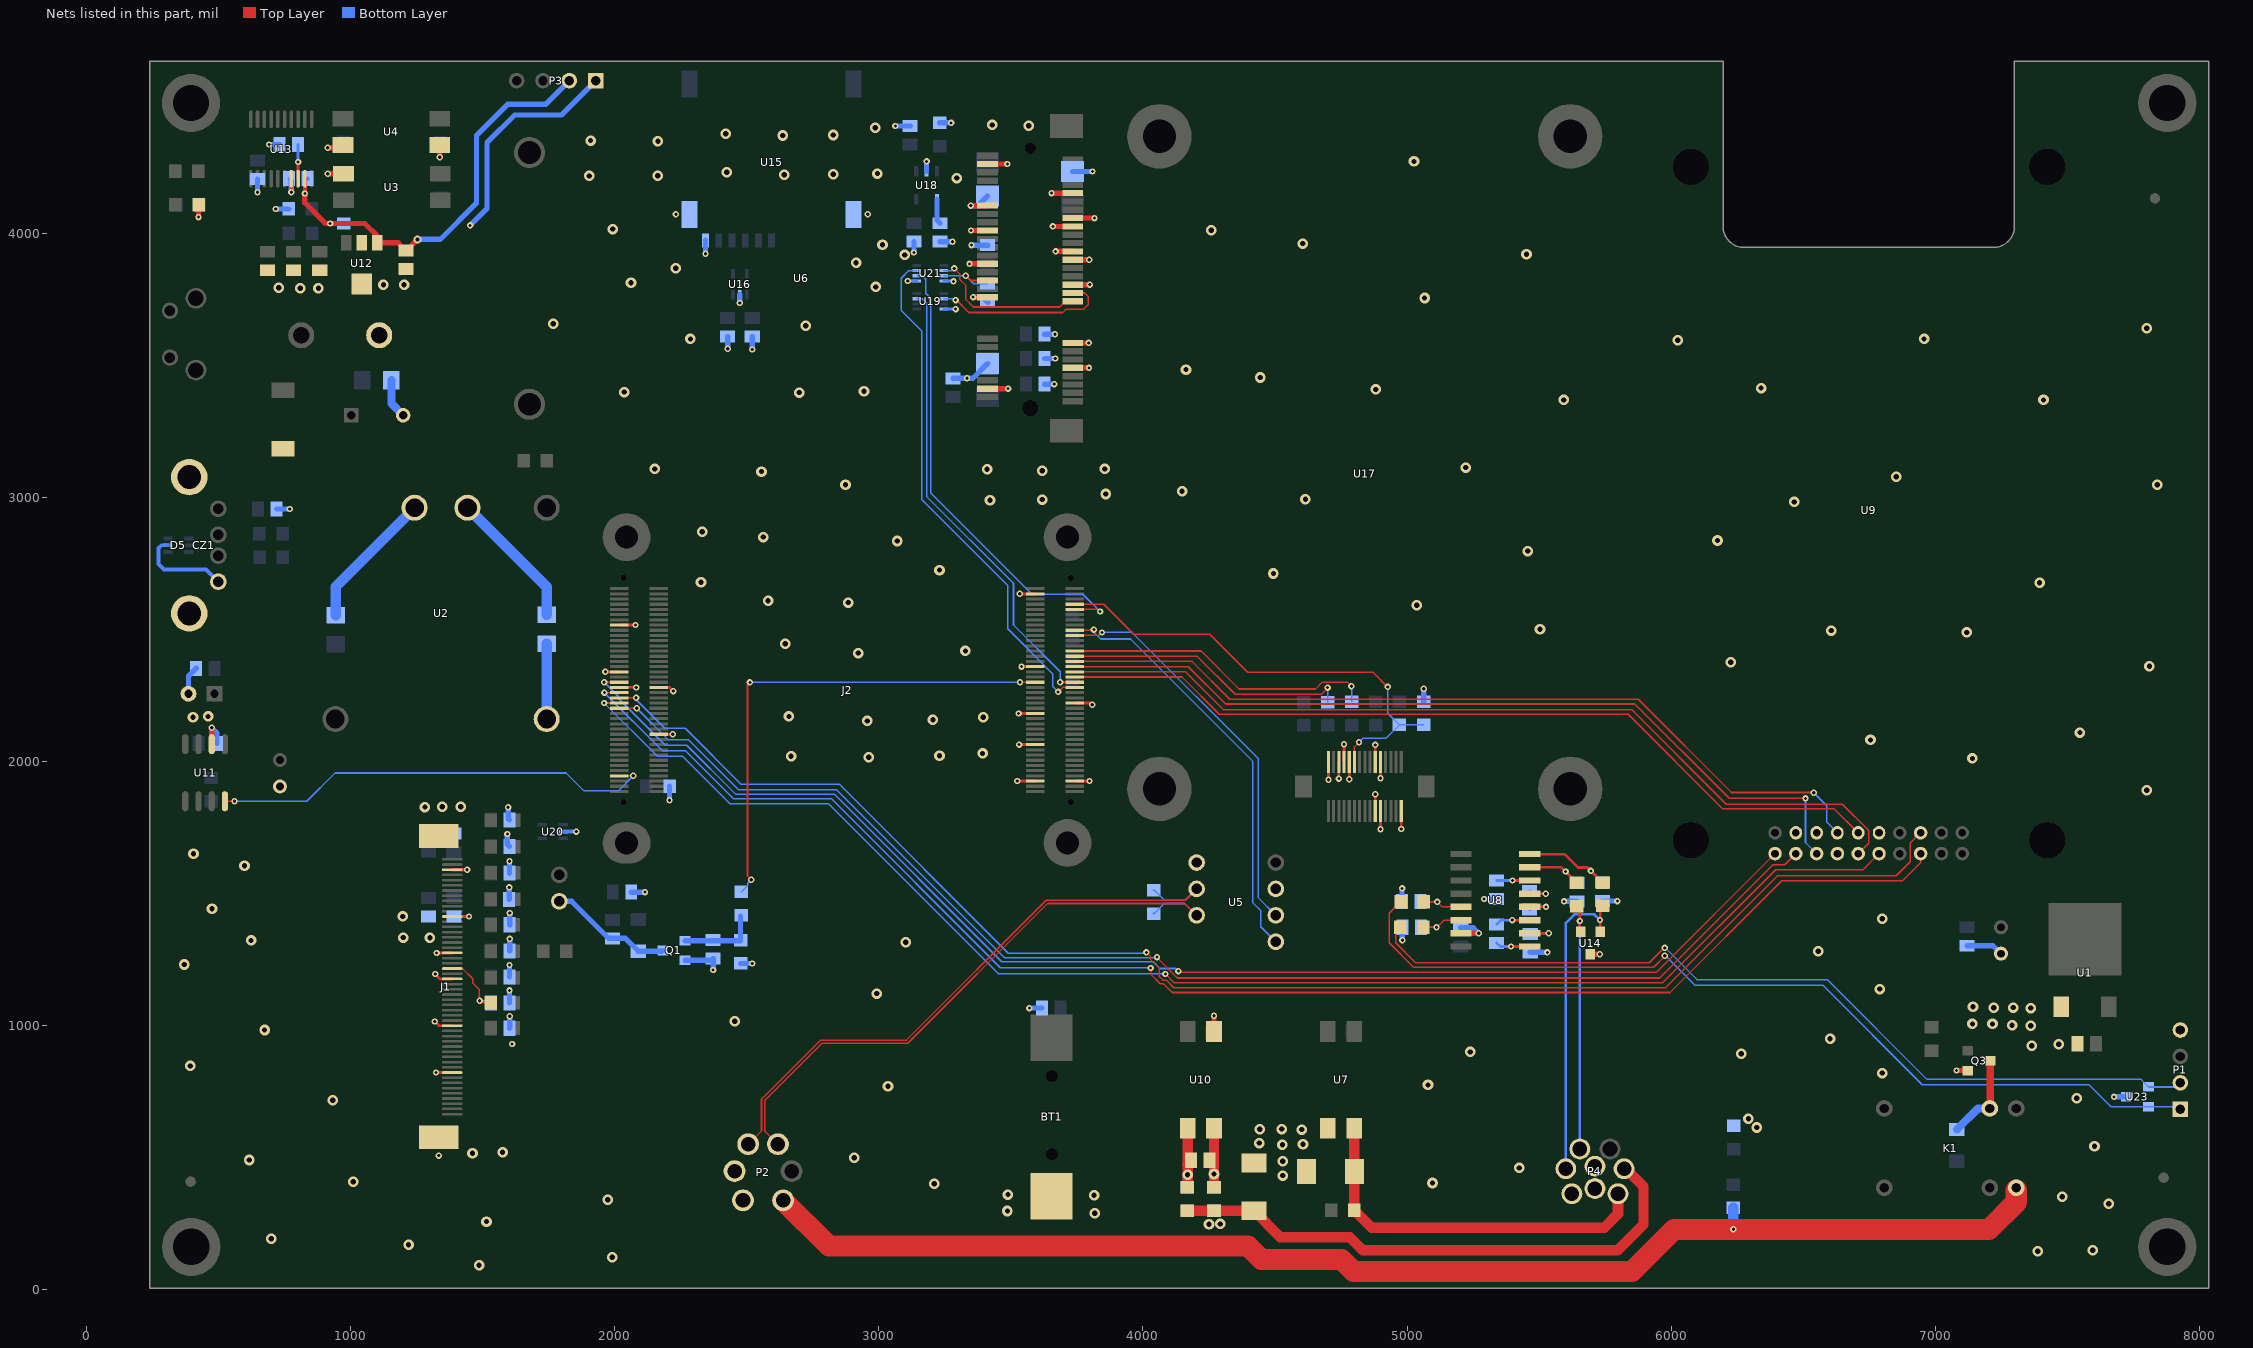
[diagram p0: the nets of this part, all layers, seen from the top]
# Altium PCB MISC82794.PcbDoc (part 3 of 5)
Units mil, origin at the board's own origin, x right, y up, seen from the top; angles counter-clockwise.
Board outline 7795.28 x 4645.67 mil, 4 copper layers (Top Layer, GND, POWER, Bottom Layer); 157 components, 133 nets, 768 pads, 456 vias.

## Part data
BT1: library part 1.10.05.0096, "2P,pitch 1.25mm,wafer with slotted frame,90°,FPC2-49T"
BZ1: library part 1.06.09.0016, "AS-905I-LF,passive,Ф9×4.8mm,Changzhou Lixiang,RoHS"
C1 C6 C27 C36 C47 C48 C49: library part 1.02.11.0018, "220μF,16V,Ф6.3×7mm,,Zhuhai Huaguan,RoHS"
C2 C4 C5 C18 C23 C30 C31 C32 C33 C34 C35 C37: library part "Cap Semi", "Capacitor (Semiconductor SIM Model)"
C3 C7 C13 C19 C22 C24 C26 C29 C50 C51 C52 C53 C54 C55 C56 C57: library part 1.02.17.0020, "0.1μF,±10%,X5R,25V,0402,RoHS"
C8 C9 C10 C11 C12: library part 1.02.17.0005, "15PF,±5%,50V,COG,0402,RoHS"
C14 C15 C16 C17: library part 1.02.17.0021, "1nF,CAP,CER,1000PF,50V,CDG,GRM1555C1H102JA01D,0402,MURATA,RoHS"
C20: library part 1.02.01.0065, "10uF,6.3V,X5R,GRM188R60J106ME47D,0603,Murata,RoHS"
C21 C28: library part 1.02.02.0055, "106,10μF,±10%,10V,X5R,0805,RoHS"
C25 C38 C39 C40 C41 C42 C43 C44 C61 C62: library part Cap, "Capacitor"
C58 C59: library part 1.02.17.0020, "1uF,±10%,X7R,25V"
C60: library part 1.02.17.0020, "22nF,±10%,X5R,50V"
CZ1: library part 1.10.12.0012, "3190004-H73-R,USB-A receptacle,vertical,90°,THT,WCON,RoHS"
D1: library part 1.04.07.0027, "1N4148,SOD-323,RoHS"
D3 D4: library part "D Zener", "Zener Diode"
D5: library part 1.05.10.0376, "NUP4202W1T2G,SC-88,ON,RoHS"
D10: library part Diode, "Default Diode"
DD1 DD2: library part LED_0
J1: library part 1.10.01.0028, "Data connector,0.5FFC-50,SMD,bottom contact,RoHS"
J2: "DF12D(3.0)-80DP-0.5V(81),Fmale,SMT,HRS,RoHS"
K1: library part Relay-SPDT, "Single-Pole Dual-Throw Relay"
L1: library part 1.03.03.0022, "BM02Y190S40R,0402,Fengjing,RoHS"
L2: library part Inductor, "Inductor"
P1 P3: library part "Header 4", "Header, 4-Pin"
P2: library part "Header 6", "Header, 6-Pin"
P4: library part "Header 8", "Header, 8-Pin"
Q1 Q3: library part 1.04.09.0001, "SS8050LT(1.5A),SOT-23,JCET,RoHS"
R1 R8 R11 R29 R30 R31 R32 R33 R34 R35 R36 R37 R38 R41 R42 R43 R44 R46 R47 R48: library part RES
R2 R3 R4 R5 R6 R25 R26: library part 1.01.17.0023, "22Ω,±5%,0402,RALEC,RoHS"
R9 R10: library part 1.01.17.0019
R12 R13 R14 R15: library part 1.01.17.0004, "0Ω,±5%,0402,RALEC,RoHS"
R16: library part "Res Varistor", "Varistor (Voltage-Sensitive Resistor)"
R17 R18 R19 R20 R21 R22 R23 R28 R49 R50: library part 1.01.17.0004
R24 R27 R39 R40 R45: library part 1.01.17.0006, "10K,±5%,0402,RALEC,RoHS"
S1: "6×6×5.0mm,black,SMD,,*"
U1 U12: library part VOLTREG1
U2: library part E2403UHBDD-10W
U3 U4 U7 U10: library part TLP281-1, "Optoisolator"
U8: library part SP202ECT
U9: library part OEMStar, "OEMStar"
U11: library part 1.05.09.0064
U14 U23: library part PESD12VL2BT
U16 U20: library part 1.05.10.0265, "PESD3V3L4UG,SOT-353,NXP,RoHS"
U18: library part RT9193, "RT9193"

## Free pads (board coordinates)
  round 39.37 smd mask+39.37: 0(395,410) 0(7831,4132) 0(7864,425)
  round 39.37 smd far side mask+39.37: 0(395,410) 0(7831,4132) 0(7864,425)

## Via types
v1: diameter 24, hole 12, Top Layer to Bottom Layer, 258 vias
v2: diameter 40, hole 20, Top Layer to Bottom Layer, 197 vias
v3: diameter 30, hole 15, Top Layer to Bottom Layer, 1 vias

## Nets (pads, with @x,y where several pads share a name; then routed paths per layer and width w, separated by ;. In a path a pad name is that pad's centre, name@x,y a point inside that pad or via, vN(x,y) a via of type N, cw(c..) or ccw(c..) an arc to the next point about the centre after c; other vN are vias at no path point)
5V: C32.1 C35.1 P3.2 R33.1 U12.1 U13.9 | length 1711.3
  Top Layer w15: v1(827.57,4150.57) U13.9@827.57,4206.79
  Top Layer w20: v1(827.57,4150.57) 827.57,4115.43 906,4037 1054,4037 1102,3989 U12.1@1102,3964.3 1180.7,3964.3 C32.1@1211,3934 v3(1254,3977)
  Bottom Layer w15: v1(827.57,4150.57) 827.57,4197.39 C35.1@836.98,4206.79
  Bottom Layer w20: v1(923,4037) R33.1@975,4037 ; v3(1254,3977) 1340,3977 1477,4114 1477,4370 1595,4488 1739,4488 P3.2@1829,4578
232RX0: P4.5 R38.1 U14.1 | length 1184.7
  Top Layer w10: U14.1@5731.4,1355.5 5731.4,1445.4 R38.1@5740,1454
  Bottom Layer w10: P4.5@5600.76,458.69 5600.76,1389.76 5633,1422 5708.4,1422 v1(5730,1400.4)
232RX1: P1.1 R48.1 U23.2 | length 3491.8
  Top Layer w6: R48.1@4954,1469 R48.1@4975,1469 4932,1426 4932,1314 5024,1222 5934,1222 5976,1264 5976,1270 5973,1267 v1(5975,1265)
  Bottom Layer w6: v1@5981,1262 6089,1154 6573,1154 6950,777 7581,777 7664.4,693.6 U23.2@7806.5,693.6 7917.4,693.6 P1.1@7927,684
232TX0: P4.4 R35.1 U14.2 | length 966.6
  Top Layer w10: R35.1@5643,1453 5654,1442 5654,1358.1 U14.2@5656.6,1355.5
  Bottom Layer w10: P4.4@5653.91,533.49 5653.91,629 v1(5653.91,1396.91)
232TX1: P1.2 R47.1 U23.1 | length 3329.1
  Top Layer w6: R47.1@4974,1373 4957,1356 4957,1314 5032,1239 5917,1239 5973.8,1295.8 v1@5973.8,1297.5 ; v1@5974.5,1297.5 v1@5973.8,1297.5 ; v1(5975,1295) 5975,1298.6 5973.8,1299.8 v1@5973.8,1297.5
  Bottom Layer w6: v1@5972,1300 6097,1175 6590,1175 6968,797 7777.9,797 U23.1@7806.5,768.4 7911.4,768.4 P1.2@7927,784
433_M0: J2.B73 R49.1 R50.1 U17.11 | length 1831
  Top Layer w6: J2.B73@3742.2,2595.8 3851.2,2595.8 3965,2482 4253,2482 4397,2338 4871,2338 v1@4927,2282 ; U17.11@4800.63,1998.52 4800.63,2055.63 v1(4818,2073)
  Bottom Layer w6: v1(4818,2073) 4833,2088 4920,2088 R49.1@4971,2139 ; v1(4927,2283) 4927,2183 R49.1@4971,2139 ; R50.1@5063,2139 R49.1@4971,2139
433_RX: J2.B53 R42.1 | length 1100.4
  Top Layer w6: J2.B53@3742.2,2398.95 4205.05,2398.95 4349,2255 4676,2255 4699,2278 v1@4699,2285
  Bottom Layer w6: v1(4699,2280) 4699,2285 4700,2286 R42.1@4700,2225
433_TX: J2.B55 R43.1 | length 1202
  Top Layer w6: J2.B55@3742.2,2418.64 4220.36,2418.64 4364,2275 4653,2275 4679,2301 4774,2301 4784,2291 4784,2285 4790,2285 v1@4789,2284 ; v1@4789,2279 v1(4789,2285)
  Bottom Layer w6: v1@4789,2279 v1(4789,2285) ; v1@4789,2284 4790,2285 R43.1@4790,2226
BOOM_SEN: D4.2 P4.2 R19.1 R20.1 | length 2074.7
  Top Layer w39.37: R20.1@4167,300 4167.55,299.45 D4.2@4421,299.45 4520.45,200 4783,200 4832,151 5798,151 5895,248 5895,391 5827.31,458.69 P4.2@5821.24,458.69
BUZZER: J2.B44 R9.1 | length 1898.7
  Top Layer w6: v1(2512,2300.06) 2503,2291.06 2503,1567 v1(2517,1553) ; v1(3534.47,2300.53) J2.B44@3592.6,2300.53
  Bottom Layer w6: R9.1@2480,1507 2504,1531 2504,1540 v1(2517,1553) ; v1(2512,2300.06) 2512.47,2300.53 v1(3534.47,2300.53)
CAN0_RXD: J2.B63 U5.1 | length 1605
  Top Layer w6: J2.B63@3742.2,2497.38 v1@3814.38,2497.38
  Bottom Layer w6: v1(3814.38,2499.62) 3814.38,2489.92 3840.3,2464 3953,2464 4415,2002 4415,1467 4446,1436 4446,1375 U5.1@4503,1318
CAN0_TXD: J2.B61 U5.2 | length 1517.8
  Top Layer w6: J2.B61@3742.2,2477.69 3833.69,2477.69 v1(3845,2489)
  Bottom Layer w6: v1(3845,2489) 3959,2489 4437,2011 4437,1484 U5.2@4503,1418
CANH0: P2.3 R32.1 U5.7 | length 2346
  Top Layer w6: P2.3@2618.3,551.81 2568,602.11 2568,717 2785,934 3110,934 3639,1463 4158,1463 U5.7@4203,1418
  Bottom Layer w6: R32.1@4040,1425 4042.4,1425 4080.4,1463 4158,1463 U5.7@4203,1418
CANL0: P2.4 R32.2 U5.6 | length 2364.3
  Top Layer w6: P2.4@2505.7,551.81 2556,602.11 2556,721.97 2780.03,946 3105.03,946 3634.03,1475 4160,1475 U5.6@4203,1518
  Bottom Layer w6: R32.2@4040,1513 4044,1513 4082,1475 4160,1475 U5.6@4203,1518
CTRL_12V: K1.2 P2.1 R39.2 | length 5014.5
  Top Layer w80: P2.1@2637.98,339.21 2811.2,166 4398,166 4449,115 4752,115 4797,70 5851,70 6010,229 7203,229 7306,332 K1.2@7306,377.4
  Bottom Layer w40: v1(6235,230) R39.2@6235,311
EN_USB0: J2.A73 U11.4 | length 1695
  Top Layer w6: U11.4@525,1849.97 v1@560.97,1849.97 ; J2.A73@2017.8,1946.2 v1(2070.8,1946.2)
  Bottom Layer w6: v1(561,1850) 835,1850 942,1957 1816,1957 1884,1889 2013.61,1889 v1(2070.8,1946.2)
GND: BT1.2 C1.2 C2.2 C3.2 C5.2 C6.2 C8.2 C9.2 C10.2 C11.2 C12.2 C13.1 C14.2 C15.2 C16.2 C17.2 C19.1 C20.1 C21.2 C22.1 C24.2 C26.1 C27.2 C28.2 C29.2 C37.2 C39.2 C40.2 C42.2 C43.2 C44.2 C47.2 C48.2 C49.2 C50.2 C51.2 C52.2 C53.2 C54.1 C55.1 C56.2 C57.2 C58.1 C59.1 C60.1 C61.1 C62.1 CZ1.4 D5.2 DD1.2 J1.3 J1.12 J1.19 J1.24 J1.33 J1.42 J1.51 J1.52 J2.A15 J2.A33 J2.A39 J2.A40 J2.A58 J2.B5 J2.B6 J2.B20 J2.B32 J2.B35 J2.B50 J2.B78 P1.4 P4.6 Q1.2 Q3.2 R10.1 R27.1 R46.2 R50.2 U1.1 U2.5 U4.3 U5.3 U6.4 U6.9 U6.15 U6.18 U6.21 U6.26 U6.27 U6.29 U6.34 U6.35 U6.37 U6.40 U6.43 U6.50 U8.15 U9.10 U9.13 U9.16 U9.18 U10.3 U11.6 U14.3 U15.5 U15.8 U15.9 U16.2 U17.1 U17.5 U17.7 U17.9 U17.19 U17.20 U17.21 U17.22 U17.30 U18.2 U19.4 U20.2 U21.4 U21.5 U23.3 | length 6377.2
  Top Layer w10: v1(1319,1016) 1334.8,1000.2 J1.33@1385.39,1000.2 ; v1(1321,1196) 1339.63,1177.37 J1.24@1385.39,1177.37 ; v1(1324.04,823.04) J1.42@1385.39,823.04 ; v1(1326.2,1275.8) J1.19@1385.39,1275.8 ; J1.12@1385.39,1413.59 v1(1448.59,1413.59) ; J2.A39@2017.8,2280.84 v1(2081.84,2280.84) ; J2.A58@2167.4,2103.68 v1(2220.32,2103.68) ; J2.A40@2167.4,2280.84 2208.16,2280.84 v1(2222,2267) ; v1(4702.2,1931.2) U17.1@4702.2,1998.52 ; v1(4741.57,1935.57) U17.5@4741.57,1998.52 ; U17.7@4761.26,1998.52 v1(4761.26,2065.74) ; v1(4780.94,1933.06) U17.9@4780.94,1998.52
  Top Layer w11: v1(1965.1,2339.9) J2.A33@2017.8,2339.9 ; J2.A15@2017.8,2517.06 v1(2079.06,2517.06) ; v1(3524.51,1926.51) J2.B6@3592.6,1926.51 ; v1(3529.42,2182.42) J2.B32@3592.6,2182.42 ; v1(3531.31,2064.31) J2.B20@3592.6,2064.31 ; v1(3533.83,2635.17) J2.B78@3592.6,2635.17 ; v1(3540.58,2359.58) J2.B50@3592.6,2359.58 ; J2.B5@3742.2,1926.51 v1(3797.49,1926.51) ; J2.B35@3742.2,2221.79 3801.21,2221.79 v1(3808,2215) ; U17.20@4879.37,1813.48 v1(4879.37,1876.37) ; U17.19@4879.37,1998.52 v1(4879.37,2063.37) ; v1(4899.06,1744.06) U17.22@4899.06,1813.48 ; v1(4899.06,1936.94) U17.21@4899.06,1998.52 ; v1(4977.8,1745.2) U17.30@4977.8,1813.48
  Top Layer w12: J1.3@1385.39,1590.76 v1(1441.76,1590.76)
  Top Layer w20: v1(425.14,4061.14) DD1.2@425.14,4108.86 ; U11.6@475,2066.03 v1(475,2128) ; v1(1338.07,4288.07) U4.3@1338.07,4334 ; v1(3343.24,3884.24) U6.26@3411.58,3884.24 ; v1(3348.28,4104.72) U6.40@3411.58,4104.72 ; v1(3349.23,4010.23) U6.34@3411.58,4010.23 ; v1(3357.26,3758.26) U6.18@3411.58,3758.26 ; U6.4@3411.58,3411.8 v1(3489.8,3411.8) ; U6.50@3411.58,4262.2 v1(3486.8,4262.2) ; v1(3654.04,4151.96) U6.43@3734.42,4151.96 ; v1(3659.02,4025.98) U6.35@3734.42,4025.98 ; v1(3669.51,3931.49) U6.29@3734.42,3931.49 ; U6.9@3734.42,3490.54 v1(3795.54,3490.54) ; U6.15@3734.42,3585.03 v1(3794.97,3585.03) ; U6.21@3734.42,3805.5 v1(3798.5,3805.5) ; U6.27@3734.42,3899.99 v1(3796.99,3899.99) ; U6.37@3734.42,4057.47 v1(3816.47,4057.47) ; U10.3@4269,978.07 v1(4269,1038) ; U8.15@5204,1350 v1(5271,1350) ; U14.3@5694,1270.5 v1(5729.5,1270.5) ; v1(7079.4,830.6) Q3.2@7122.5,830.6
  Bottom Layer w10: U21.4@3246.18,3819.47 3281.53,3819.47 v1(3283,3818)
  Bottom Layer w11: v1(3109.47,3819.47) U21.5@3143.82,3819.47 ; U19.4@3246.45,3712.94 v1(3290.94,3712.94)
  Bottom Layer w15: D5.2@309.55,2819 285,2819 274,2808 274,2748 294,2728 453.32,2728 CZ1.4@500.12,2681.2 ; U20.2@1805.45,1735 v1(1855,1735)
  Bottom Layer w20: C27.2@386.79,2257 386.79,2323.79 C28.2@416,2353 ; v1(475,2128) 495,2108 C26.1@495,2069 ; C29.2@720,2956 v1(770,2956) ; v1(1594,1726) 1594,1686.6 C15.2@1602,1678.6 ; v1(1597,1827) 1597,1783.6 C17.2@1602,1778.6 ; C14.2@1601,1478.6 v1(1601,1524) ; C11.2@1602,990.6 1603,991.6 v1(1603,1036) ; C10.2@1602,1086.6 v1(1602,1134) ; C12.2@1602,1184.6 v1(1602,1230) ; C16.2@1602,1577.6 v1(1602,1623) ; C9.2@1603,1283 v1(1603,1329) ; C8.2@1603,1382.6 v1(1603,1427) ; C3.2@2063,1506 v1(2115,1506) ; v1(2208,1854) R27.1@2208,1907 ; Q1.2@2266.5,1247.6 C13.1@2366.6,1247.6 ; v1(2344.39,3922.39) U15.5@2344.39,3973.23 ; v1(2373,1211) C13.1@2373,1254 ; v1(2428,3563) C55.1@2428,3609 ; v1(2474,3736) U16.2@2474,3767.55 ; R10.1@2478,1236 v1(2521,1236) ; v1(2521,3560) C54.1@2521,3609 ; v1(3063,4406) C59.1@3119,4406 ; v1(3133,3927) C58.1@3133,3968 ; U18.2@3181,4235.15 v1(3181,4272) ; R46.2@3230,4418 v1(3274,4418) ; C60.1@3232,3968 v1(3279,3968) ; C57.2@3281,3451 v1(3334,3451) 3356.01,3451 C48.2@3412,3506.99 ; v1(3348.28,4104.72) 3374.71,4104.72 C47.2@3411,4141.01 ; v1(3351,3955) C56.2@3412,3955 ; v1(3357.26,3758.26) 3392.74,3758.26 C53.2@3412,3739 ; v1(3570,1067) C24.2@3618,1067 ; C50.2@3627,3429 v1(3664,3429) ; C51.2@3627,3526 v1(3668,3526) ; C52.2@3627,3618 v1(3667,3618) ; C49.2@3734,4233.99 v1(3808.99,4233.99) ; C62.1@4981,1470 v1(4981,1520) ; v1(4982,1324) C61.1@4982,1373 ; R50.2@5063,2227 v1(5063,2276) ; C39.2@5203,1371 5250,1371 v1(5271,1350) ; v1(5291,1480) C42.2@5339,1480 ; C40.2@5466,1278 v1(5531,1278) ; v1(5594,1471) C44.2@5643,1471 ; C43.2@5740,1472 v1(5796,1472) ; C5.2@7120,1303 7218,1303 C1.2@7248,1273 ; v1(7676,731) U23.3@7721.5,731
  Bottom Layer w40: U2.5@1743,2161 C37.2@1743,2445.88
  other v1: 1334.61,508.39 1612,931 2231.85,4071.85 2958.15,4071.85
  other v2: 1487,94 1991,124 7387,147 7595,150 1220,171 700,194 1515,259 3818,290 3487,299 7656,326 1974,342 7480,353 3815,359 3489,361 3210,402 5096,405 1011,410 5425,462 617,492 2907,500 1462,518 1576,521 7602,544 933,718 7535,726 3035,771 5079,776 6799,821 394,848 6265,894 5239,901 7364,924 7467,930 6601,951 675,984 7361,1000 7290,1002 7140,1007 7216,1007 2455,1017 7361,1067 7221,1068 7295,1069 7142,1072 2992,1122 6789,1139 371,1232 6556,1282 3102,1316 624,1323 1301,1333 1200,1334 6799,1405 1198,1414 476,1443 599,1606 406,1651 1282,1828 1348,1829 1418,1829 7800,1892 7140,2012 2962,2017 2668,2020 3230,2022 3393,2031 6754,2082 7547,2110 2956,2154 3205,2159 404,2168 3396,2168 461,2171 2660,2171 7810,2361 6225,2376 2922,2411 3328,2419 2646,2446 7118,2489 6606,2496 5503,2501 5036,2592 2884,2602 2581,2609 7394,2677 2327,2679 4494,2712 3230,2725 5457,2797 3070,2835 6175,2837 2563,2850 2332,2870 6466,2983 3421,2989 3619,2992 4615,2993 3859,3013 4148,3023 2874,3048 7840,3048 6852,3078 2556,3098 3619,3101 3410,3107 2152,3108 3855,3108 5222,3113 5593,3369 7409,3369 2699,3397 2036,3399 2944,3402 4881,3409 6340,3414 4444,3454 4163,3484 6024,3595 2287,3600 6957,3600 7800,3640 2724,3650 1768,3658 5066,3755 2989,3797 2062,3813 2231,3868 2914,3888 3098,3918 5452,3921 3014,3957 4605,3961 4259,4011 1993,4016 3295,4209 1904,4217 2163,4218 2642,4221 2828,4223 2995,4226 2425,4231 5026,4272 2164,4348 1909,4351 2637,4370 2828,4372 2421,4377 2987,4399 3568,4407 3430,4410
GND1: C18.2 C23.1 C30.2 C31.2 C32.2 C33.1 C34.1 C35.2 C36.2 C37.1 CZ1.5 CZ1.6 D3.1 D4.1 P2.5 P2.6 P3.1 P4.7 P4.8 R16.1 R23.2 R34.1 R40.2 U2.2 U3.3 U4.2 U5.5 U7.3 U12.2 U13.7 | length 1898.1
  Top Layer w12: v1(776.39,4155.39) U13.7@776.39,4206.79
  Top Layer w20: v1(914,4225) U3.3@973.93,4225 ; v1(914,4324) 961.93,4324 U4.2@971.93,4334
  Bottom Layer w12: C35.2@766.98,4206.79 C35.2@776.39,4197.38
  Bottom Layer w20: v1(648,4155) C34.1@648,4205 ; v1(692,4336) C33.1@732,4336 ; v1(717,4092) R34.1@766,4092 ; v1(776.39,4155.39) C35.2@776.39,4197.38 ; v1@1453,4029 v1(1453,4030) 1517,4094 1517,4343 1622,4448 1799,4448 P3.1@1929,4578
  Bottom Layer w30: C23.1@1155.12,3444 1155.12,3355.31 C36.2@1199.43,3311
  Bottom Layer w40: U2.2@1443,2961 1743,2661 C37.1@1743,2556.12
  other v2: 4250,249 4293,250 4529,433 4529,487 4528,550 4606,552 4440,556 4601,607 4442,608 4525,609 6324,615 6292,648 810,3792 879,3792 729,3794 1125,3805 1203,3805
GND_SPD: D3.2 P4.1 R17.1 U7.4 | length 1433.2
  Top Layer w40: U7.4@4800,611.93 R17.1@4800,302 4866,236 5746,236 5798.4,288.4 P4.1@5798.4,364.2
GPS_EVT1: J2.A45 U9.9 | length 5525.6
  Top Layer w6: v1(1960.21,2221.79) J2.A45@2017.8,2221.79 ; v1(4085,1196) 4118,1163 5967,1163 6395,1591 6725.58,1591 U9.9@6786.39,1651.8
  Bottom Layer w6: v1(1960.21,2221.79) 2161,2021 2256,2021 2437,1840 2810,1840 3453,1197 4082,1197 4084,1195 v1(4085,1196)
GPS_PPS: J2.A37 U9.19 | length 5129.9
  Top Layer w6: v1(1960.47,2300.53) J2.A37@2017.8,2300.53 ; v1@4138,1202 5942.88,1202 U9.19@6392.69,1651.8
  Bottom Layer w6: v1(1960.47,2300.53) 2014,2247 2014,2240 2192,2062 2273,2062 2458,1877 2831,1877 3466,1242 4040,1242 4065,1217 4124,1217 v1(4134,1207) v1@4134,1206
GPS_PV: J2.A47 U9.17 | length 5070.8
  Top Layer w6: J2.A47@2017.8,2202.1 v1(2083.9,2202.1) ; v1(4053,1260) 4053,1258.3 4130.3,1181 5956,1181 6385,1610 6429.62,1610 U9.17@6471.43,1651.8
  Bottom Layer w6: v1(2083.9,2202.1) 2204,2082 2281,2082 2469,1894 2840,1894 3477,1257 v1@4050,1257
GPS_RST: J2.A41 U9.5 | length 5760.7
  Top Layer w6: v1(1961.16,2261.16) J2.A41@2017.8,2261.16 ; v1(4029,1219) 4029,1196 4066,1159 4078,1159 4111,1126 5995,1126 6418,1549 6875,1549 6943.87,1617.87 U9.5@6943.87,1651.8
  Bottom Layer w6: v1(1961.16,2261.16) 2181.32,2041 2268,2041 2449,1860 2820,1860 3460,1220 4028,1220 v1(4029,1219)
GPS_RX1: J2.B45 U9.12 | length 3209.7
  Top Layer w6: J2.B45@3742.2,2320.21 4147.79,2320.21 4289,2179 5837,2179 6195,1821 6617.19,1821 U9.12@6707.65,1730.54
GPS_RX2: J2.B49 U9.15 | length 3199
  Top Layer w6: J2.B49@3742.2,2359.58 4171.42,2359.58 4313,2218 5862,2218 6219,1861 v1(6508,1861)
  Bottom Layer w6: v1(6508,1861) 6508,1693.97 U9.15@6550.17,1651.8
GPS_TX1: J2.B47 U9.11 | length 3357.4
  Top Layer w6: J2.B47@3742.2,2339.9 4161.1,2339.9 4304,2197 5850,2197 6208,1839 6647.29,1839 6747,1739.29 6747,1691.16 U9.11@6707.65,1651.8
GPS_TX2: J2.B51 U9.14 | length 3192.1
  Top Layer w6: J2.B51@3742.2,2379.27 4185.73,2379.27 4329,2236 5875,2236 6228,1883 v1@6540,1883
  Bottom Layer w6: v1(6539,1882) 6588,1833 6588,1771.45 U9.14@6628.91,1730.54
GPS_VARF: J2.A43 U9.6 | length 5696.2
  Top Layer w6: J2.A43@2017.8,2241.47 v1(2081.47,2241.47) ; v1(4013,1278) 4027,1264 4027,1253 4061,1219 4061,1188 4076,1173 4088,1173 4117,1144 5978,1144 6402,1568 6852,1568 6905,1621 6905,1691.68 U9.6@6943.87,1730.54
  Bottom Layer w6: v1(2081.47,2241.47) 2081.47,2234.53 2190,2126 2267,2126 2478,1915 2850,1915 3490,1275 4010,1275 v1(4013,1278)
HSYNC: C10.1 J1.22 R4.2 | length 266.1
  Top Layer w6: J1.22@1385.39,1216.74 1424.26,1216.74 1463.4,1177.6 1463.4,1162.27 1488,1137.67 v1@1488,1096 ; v1@1497.4,1086.6 R4.2@1531,1086.6
  Bottom Layer w6: v1(1489,1095) 1523.6,1095 C10.1@1532,1086.6
LTE_RST: J2.B71 U21.6 | length 1782.1
  Top Layer w6: J2.B71@3742.2,2576.12 3829.88,2576.12 v1(3838,2568)
  Bottom Layer w6: U21.6@3143.82,3839.16 3163.84,3839.16 3177.5,3825.5 3177.5,3772.5 3196,3754 3196,3018 3580.14,2633.86 3772.14,2633.86 v1(3838,2568)
LTE_RST1.8: C53.1 U6.22 U21.3 | length 283.1
  Top Layer w6: v1(3329,3839) 3346.75,3821.25 U6.22@3411.58,3821.25
  Bottom Layer w6: U21.3@3246.18,3839.16 3272,3839.16 ; 3286.84,3839.16 3272,3839.16 ; C53.1@3412,3809 3360,3809 3330,3839 v1(3329,3839) 3328.84,3839.16 3272,3839.16
LTE_RX: J2.B41 U21.7 | length 1954.2
  Top Layer w6: v1@3679.7,2264 3696.54,2280.84 J2.B41@3742.2,2280.84 J2.B41@3740.89,2279.53
  Bottom Layer w6: U21.7@3143.82,3858.84 3113.84,3858.84 3085,3830 3085,3708 3162,3631 3162,2993 3488,2667 3488,2503 3659,2332 3659,2284 v1(3679,2264)
LTE_RX1.8: U6.17 U21.2 | length 595.5
  Top Layer w6: U6.17@3734.42,3742.51 3706.51,3742.51 3685,3721 3358,3721 3330,3749 3330,3802 3306,3826 3306,3847 v1@3286.5,3866.5 ; v1@3286.5,3866.5 v1(3286,3867) 3287,3867 v1@3286.5,3866.5
  Bottom Layer w6: U21.2@3246.18,3858.84 v1@3278.84,3858.84
LTE_TX: J2.B43 U19.7 | length 1744.2
  Top Layer w6: v1(3686.53,2300.53) J2.B43@3742.2,2300.53
  Bottom Layer w6: U19.7@3144.08,3752.31 3164.69,3752.31 3181,3736 3181,3004 3510,2675 3510,2517 3686.53,2340.47 v1(3686.53,2300.53)
LTE_TX1.8: U6.19 U19.2 | length 675.3
  Top Layer w6: v1(3291,3747) 3291,3750 3341,3700 3697,3700 3709,3712 3775,3712 3793,3730 3793,3761 3779.99,3774.01 U6.19@3734.42,3774.01
  Bottom Layer w6: U19.2@3246.45,3752.31 v1@3288.69,3752.31
NetBZ1_2: BZ1.2 C7.1 D1.1 Q1.3 | length 470
  Bottom Layer w20: BZ1.2@1791,1471 1838,1471 1978,1331 2041,1331 D1.1@2090,1282 2178.5,1282 Q1.3@2181.5,1285
NetC4_1: C4.1 L2.2 U2.1 | length 530.7
  Bottom Layer w40: C4.1@944,2554.12 944,2662 U2.1@1243,2961
NetC13_2: C13.2 Q1.1 R9.2 R10.2 | length 302.9
  Bottom Layer w20: Q1.1@2266.5,1322.4 2476.4,1322.4 R9.2@2476.4,1415.4
NetC25_1: C25.1 R20.2 R22.1 U10.1 | length 317
  Top Layer w39.37: R20.2@4167,388 4169,390 U10.1@4169,611.93 ; C25.1@4167,475 4183,491 C25.1@4169,505
  Bottom Layer w39.37: R22.1@4167,388 4169,390 v2@4169,437
  other v2: 4169,436
NetC25_2: C25.2 R19.2 R23.1 U10.2 | length 320.2
  Top Layer w39.37: R19.2@4269,388 U10.2@4269,611.93 ; C25.2@4269,475 4253,491 C25.2@4269,507
  Bottom Layer w39.37: R23.1@4269,388 v2(4269,439)
NetC33_2: C33.2 U13.8 | length 129.2
  Top Layer w11.81: U13.8@801.98,4206.79 v1(801.98,4269.98)
  Bottom Layer w11.81: v1@802,4270 C33.2@802,4336
NetC38_1: C38.1 U8.3 | length 131.6
  Top Layer w10: v1(5398,1400) U8.3@5464,1400
  Bottom Layer w10: C38.1@5339,1384 5355,1400 v1(5398,1400)
NetC38_2: C38.2 U8.1 | length 130.8
  Top Layer w10: v1(5393,1300) U8.1@5464,1300
  Bottom Layer w10: C38.2@5339,1314 5353,1300 v1(5393,1300)
NetC40_1: C40.1 U8.2 | length 142.8
  Top Layer w10: U8.2@5464,1350 v1(5536,1350)
  Bottom Layer w10: C40.1@5466,1348 5468,1350 v1(5536,1350)
NetC41_1: C41.1 U8.5 | length 126.1
  Top Layer w10: U8.5@5464,1500 v1(5525,1500)
  Bottom Layer w10: C41.1@5464,1510 5474,1500 v1(5525,1500)
NetC41_2: C41.2 U8.4 | length 128.1
  Top Layer w10: U8.4@5464,1450 v1(5526,1450)
  Bottom Layer w10: C41.2@5464,1440 5474,1450 v1(5526,1450)
NetC42_1: C42.1 U8.6 | length 125
  Top Layer w10: v1(5399,1550) U8.6@5464,1550
  Bottom Layer w10: C42.1@5339,1550 v1(5399,1550)
NetC43_1: C43.1 R38.2 U8.8 | length 383.7
  Top Layer w10: U8.8@5464,1650 5596,1650 5647,1599 5683,1599 v1(5695.5,1586.5) R38.2@5740,1542
  Bottom Layer w10: v1(5695.5,1586.5) C43.1@5740,1542
NetC44_1: C44.1 R35.2 U8.7 | length 264.2
  Top Layer w10: U8.7@5464,1600 5584,1600 v1(5600,1584) R35.2@5643,1541
  Bottom Layer w10: v1(5600,1584) C44.1@5643,1541
NetC60_2: C60.2 U18.4 | length 95.7
  Bottom Layer w20: U18.4@3220.37,4128.85 3220.37,4049.63 C60.2@3232,4038
NetC61_2: C61.2 R47.2 U8.14 | length 212.2
  Top Layer w6: R47.2@5062,1373 v1(5111,1373) 5113,1373 5140,1400 U8.14@5204,1400
  Bottom Layer w6: C61.2@5052,1373 v1(5111,1373)
NetC62_2: C62.2 R48.2 U8.13 | length 212.3
  Top Layer w6: R48.2@5063,1469 v1(5114,1469) 5133,1450 U8.13@5204,1450
  Bottom Layer w6: C62.2@5051,1470 5113,1470 v1(5114,1469)
NetD10_1: D10.1 K1.5 Q3.3 | length 337.6
  Top Layer w30: K1.5@7207.5,688.5 Q3.3@7207.5,868
  Bottom Layer w30: D10.1@7081,607 7161,687 K1.5@7206,687